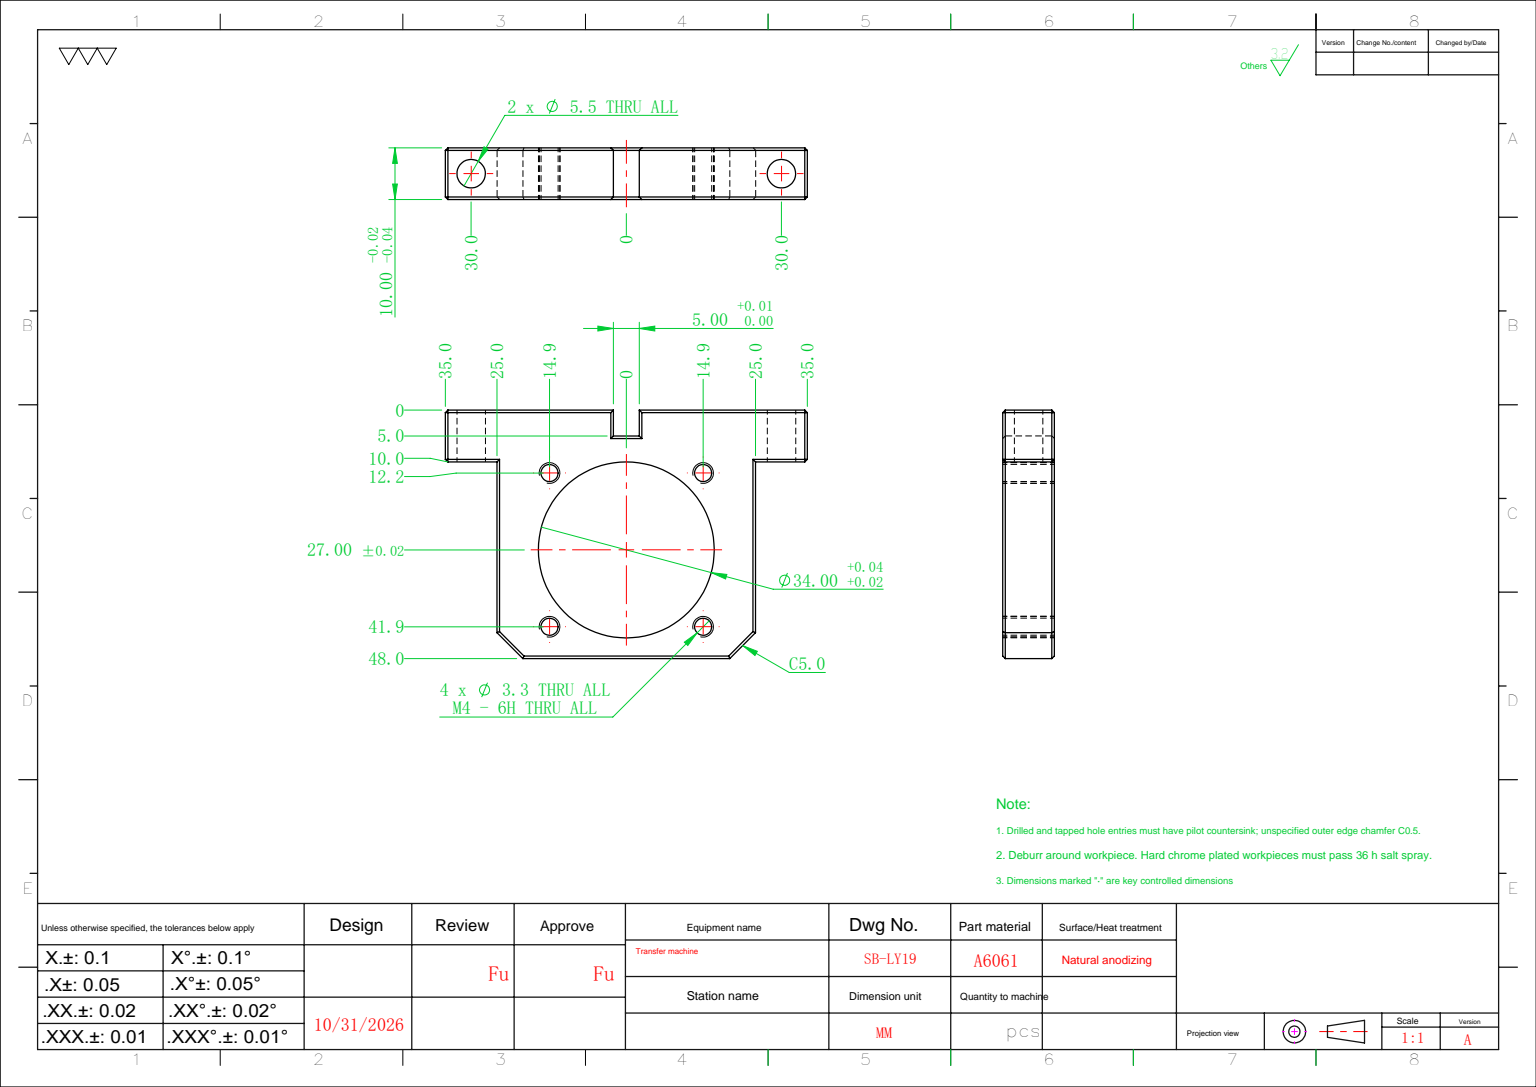
SolidWorks part; units mm, degrees
ref_plane "前视基准面" through (0, 0, 0) normal (0, 0, 1) x (1, 0, 0)
ref_plane "上视基准面" through (0, 0, 0) normal (0, 1, 0) x (1, 0, 0)
ref_plane "右视基准面" through (0, 0, 0) normal (1, 0, 0) x (0, 0, -1)
sketch "草图1" plane through (0, 0, 0) normal (0, 0, 1) x (1, 0, 0)
  line L1 (-35, -24) -> (35, -24)
  line L2 (-35, -24) -> (-35, 24)
  line L3 (-35, 24) -> (35, 24)
  line L4 (35, -24) -> (35, 24)
  line L5 (-35, -24) -> (35, 24) construction
  line L6 (-35, 24) -> (35, -24) construction
  point P0 (0, 0)
  dimension "D1" = 70
  dimension "D2" = 48
extrude "凸台-拉伸1" add sketch "草图1" along normal blind 10
sketch "草图2" plane through (0, 0, 10) normal (0, 0, 1) x (1, 0, 0)
  line L0 (0, 0) -> (0, -35.8295) construction
  line L1 (-35, -24) -> (-25, -24)
  line L2 (-35, -24) -> (-35, 14)
  line L3 (-35, 14) -> (-25, 14)
  line L4 (-25, -24) -> (-25, 14)
  line L5 (25, -24) -> (25, 14)
  line L6 (35, 14) -> (25, 14)
  line L7 (35, -24) -> (35, 14)
  line L8 (35, -24) -> (25, -24)
  line L9 (35, 24) -> (-35, 24) construction
  dimension "D1" = 10
  dimension "D2" = 10
extrude "切除-拉伸1" cut sketch "草图2" against normal through all
sketch "草图3" plane through (0, 0, 0) normal (0, 0, -1) x (-1, 0, 0)
  line L0 (0, 0) -> (0, -40.7468) construction
  line L1 (-35, 24) -> (35, 24) construction
  circle A0 centre (0, -3) radius 17
  dimension "D1" = 34
  dimension "D2" = 27
extrude "切除-拉伸2" cut sketch "草图3" against normal through all
hole_wizard "M4 螺纹孔2" positions "草图8" profile "草图9" tap size "M4" standard "ISO" end condition through all
sketch "草图8" plane through (0, 0, 10) normal (0, 0, 1) x (1, 0, 0)
  line L0 (0, -3) -> (0, -34.3856) construction
  line L3 (0, -3) -> (-29.4307, -3) construction
  point P0 (14.85, -17.85)
  point P2 (-14.85, -17.85)
  point P4 (-14.85, 11.85)
  point P6 (14.85, 11.85)
  dimension "D1" = 29.7
  dimension "D2" = 29.7
sketch "草图9" plane through (14.85, -17.85, 10) normal (1, 0, 0) x (0, -1, 0)
  line L0 (0, 0) -> (0, 10)
  line L1 (0, 10) -> (1.65, 10)
  line L2 (1.65, 10) -> (1.65, 0)
  line L5 (1.65, 0) -> (0, 0)
  line L11 (0, -6.35) -> (0, 107.95) construction
  dimension "通孔螺纹孔钻头直径" = 3.3
  dimension "通孔螺纹孔钻头深度" = 10
cosmetic thread "孔螺蚊线5" parameters "D2"=4
cosmetic thread "孔螺蚊线6" parameters "D2"=4
cosmetic thread "孔螺蚊线7" parameters "D2"=4
cosmetic thread "孔螺蚊线8" parameters "D2"=4
hole_wizard "Ø5.5 (5.5) 直径孔1" positions "草图10" profile "草图11" hole size "Ø5.5" standard "ISO" end condition through all
sketch "草图10" plane through (0, 14, 0) normal (0, -1, 0) x (-1, 0, 0)
  line L0 (35, -5) -> (-35, -5) construction
  line L1 (35, 0) -> (35, -10) construction
  line L2 (-35, 0) -> (-35, -10) construction
  line L4 (0, 0) -> (0, -15.7163) construction
  point P0 (-30, -5)
  point P2 (30, -5)
  dimension "D1" = 60
sketch "草图11" plane through (30, 14, 5) normal (1, 0, 0) x (0, 0, -1)
  line L0 (0, 0) -> (0, 10)
  line L1 (0, 10) -> (2.75, 10)
  line L2 (2.75, 10) -> (2.75, 0)
  line L5 (2.75, 0) -> (0, 0)
  line L11 (0, -6.35) -> (0, 107.95) construction
  dimension "通孔孔直径" = 5.5
  dimension "通孔孔深度" = 10
chamfer "倒角1" distance 5 angle 45 2 edges at (-25, -24, 5) (25, -24, 5)
sketch "草图12" plane through (0, 0, 10) normal (0, 0, 1) x (1, 0, 0)
  line L0 (35, 24) -> (-35, 24) construction
  line L1 (-2.5, 24) -> (2.5, 24)
  line L2 (-2.5, 24) -> (-2.5, 19)
  line L3 (-2.5, 19) -> (2.5, 19)
  line L4 (2.5, 24) -> (2.5, 19)
  line L5 (0, 0) -> (0, 36.1087) construction
  dimension "D1" = 5
  dimension "D2" = 5
extrude "切除-拉伸3" cut sketch "草图12" against normal through all
chamfer "倒角2" distance 0.5 angle 45 32 edges at (-18.75, 24, 0) (-30, 14, 0) (-25, -2.5, 0) (-22.5, -21.5, 0) (0, -24, 0) (22.5, -21.5, 0) (25, -2.5, 0) (30, 14, 0) (-2.5, 21.5, 0) (0, 19, 0) (2.5, 21.5, 0) (18.75, 24, 0) (2.5, 21.5, 10) (18.75, 24, 10) (0, 19, 10) (-2.5, 21.5, 10) (-18.75, 24, 10) (-35, 24, 5) (-35, 19, 10) (-35, 19, 0) (-35, 14, 5) (-30, 14, 10) (-25, -2.5, 10) (-22.5, -21.5, 10) (0, -24, 10) (22.5, -21.5, 10) (25, -2.5, 10) (30, 14, 10) (35, 24, 5) (35, 19, 0) (35, 14, 5) (35, 19, 10)
